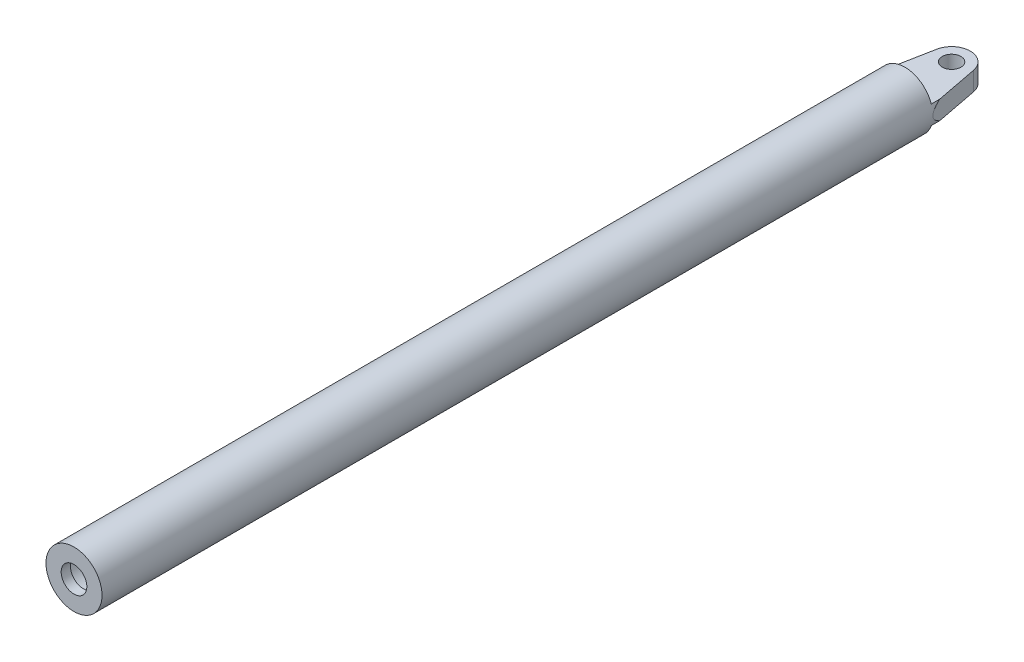
SolidWorks part; units mm, degrees
material "1.0503 (C45)"
ref_plane "前视基准面" through (0, 0, 0) normal (0, 0, 1) x (1, 0, 0)
ref_plane "上视基准面" through (0, 0, 0) normal (0, 1, 0) x (1, 0, 0)
ref_plane "右视基准面" through (0, 0, 0) normal (1, 0, 0) x (0, 0, -1)
sketch "草图1" plane through (0, 0, 0) normal (0, 0, 1) x (1, 0, 0)
  circle A0 centre (0, 0) radius 60
  circle A1 centre (0, 0) radius 45
  dimension "D1" = 120
  dimension "D2" = 15
extrude "凸台-拉伸1" add sketch "草图1" along normal blind 1780
sketch "草图2" plane through (0, 0, 0) normal (0, 1, 0) x (1, 0, 0)
  line L0 (0, 0) -> (0, 100) construction
  line L1 (45, 0) -> (-45, 0) construction
  line L2 (-60, 0) -> (-39.2778, 107.5667)
  line L3 (60, 0) -> (39.2778, 107.5667)
  line L4 (-60, 0) -> (60, 0)
  circle A0 centre (0, 100) radius 20
  arc A1 (39.2778, 107.5667) -> (-39.2778, 107.5667) centre (0, 100) ccw
  dimension "D1" = 40
  dimension "D2" = 80
  dimension "D3" = 100
extrude "凸台-拉伸2" add sketch "草图2" along normal mid plane 40
sketch "草图3" plane through (0, 0, 0) normal (0, 0, -1) x (-1, 0, 0)
  circle A1 centre (0, 0) radius 50
  dimension "D1" = 100
extrude "凸台-拉伸3" add sketch "草图3" against normal blind 40
sketch "草图4" plane through (0, 0, 0) normal (0, 0, -1) x (-1, 0, 0)
  circle A0 centre (0, 0) radius 60
  dimension "D1" = 120
extrude "切除-拉伸1" cut sketch "草图4" along normal through all flip side to cut
sketch "草图5" plane through (0, 0, 1780) normal (0, 0, 1) x (1, 0, 0)
  circle A0 centre (0, 0) radius 27.5
  circle A2 centre (0, 0) radius 60
  circle A3 centre (0, 0) radius 60
  dimension "D1" = 55
  dimension "D2" = 0
extrude "凸台-拉伸4" add sketch "草图5" against normal blind 20
